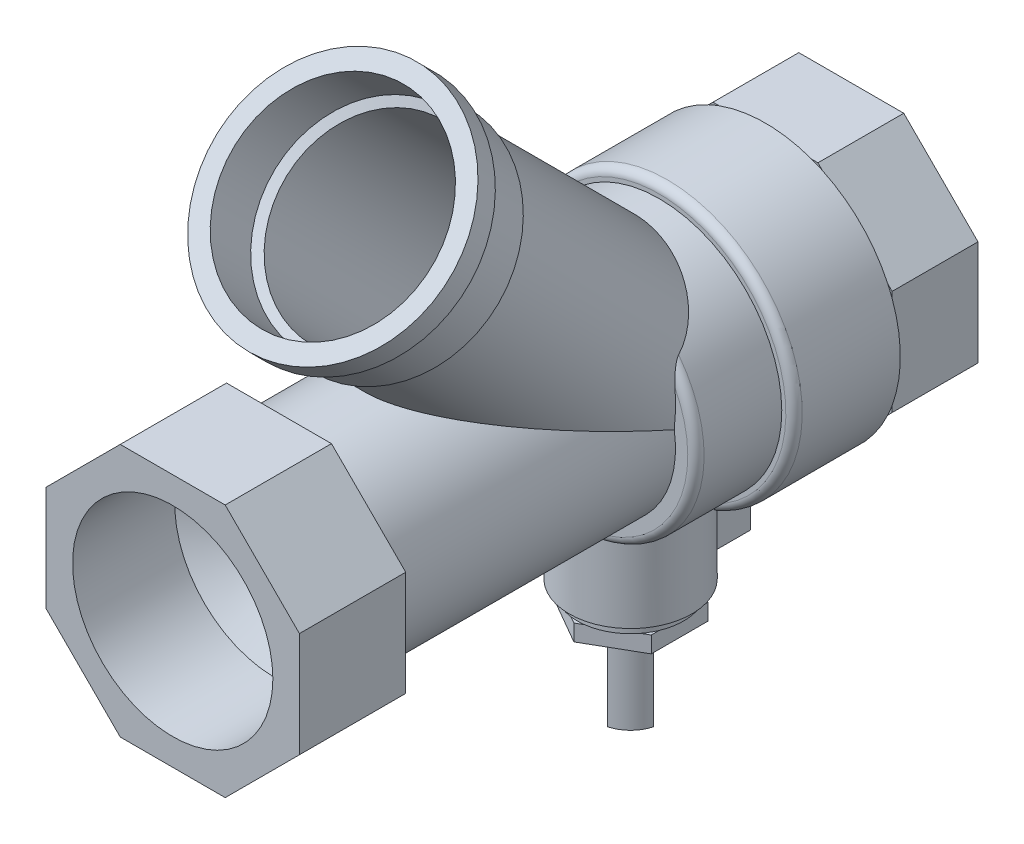
from build123d import *

# Parameters (mm, degrees)
SKETCH_1_R               = 15
EXTRUDE_1_DEPTH          = 10.5
SKETCH_2_R               = 12.5
EXTRUDE_2_DEPTH          = 36
EXTRUDE_3_DEPTH          = 13
SKETCH_4_R               = 16.5
EXTRUDE_4_DEPTH          = 13
EXTRUDE_5_DEPTH          = 10.5
FILLET_1_R               = 1
HOLE_WIZARD_G3_4_1_D     = 24.5
HOLE_WIZARD_G3_4_1_DEPTH = 12.5
HOLE_WIZARD_G3_4_1_TIP   = 7.360542583
HOLE_WIZARD_G3_4_2_D     = 24.5
HOLE_WIZARD_G3_4_2_DEPTH = 12.5
HOLE_WIZARD_G3_4_2_TIP   = 7.360542583
EXTRUDE_6_REACH          = 75.57
SKETCH_13_R              = 6.5
EXTRUDE_7_DEPTH          = 1.25
EXTRUDE_8_DEPTH          = 2
SKETCH_15_R              = 4
EXTRUDE_9_DEPTH          = 10
SKETCH_18_R              = 12.5
SKETCH_19_R              = 13.25
EXTRUDE_10_DEPTH         = 7
SKETCH_20_R              = 14.5
EXTRUDE_11_DEPTH         = 3
HOLE_WIZARD_G3_4_3_D     = 24.5
HOLE_WIZARD_G3_4_3_DEPTH = 7
HOLE_WIZARD_G3_4_3_TIP   = 7.360542583
SKETCH_24_R              = 11.25
CUT_EXTRUDE_2_DEPTH      = 45
CUT_EXTRUDE_1_REACH      = 97.54
SKETCH_11_R              = 7.5
CUT_EXTRUDE_START        = -10
CUT_EXTRUDE_3_DEPTH      = 10


with BuildPart() as part:
    # 草图1 → 凸台-拉伸1 (new body)
    with BuildSketch(Plane.XY):
        with Locations(Location((0, 0, 0), (0, 0, 180))):
            Circle(SKETCH_1_R)
    extrude(amount=EXTRUDE_1_DEPTH)

    # 草图2 → 凸台-拉伸2 (add)
    with BuildSketch(Plane.XY.offset(10.5)):
        Circle(SKETCH_2_R)
    extrude(amount=EXTRUDE_2_DEPTH)

    # 草图3 → 凸台-拉伸3 (add)
    with BuildSketch(Plane.XY.offset(46.5)):
        Polygon((6.420310217, -15.5), (15.5, -6.420310217), (15.5, 6.420310217), (6.420310217, 15.5), (-6.420310217, 15.5), (-15.5, 6.420310217), (-15.5, -6.420310217), (-6.420310217, -15.5), align=None)
    extrude(amount=EXTRUDE_3_DEPTH)

    # 草图4 → 凸台-拉伸4 (add)
    with BuildSketch(Plane(origin=(0, 0, 0), x_dir=(-1, 0, 0), z_dir=(0, 0, -1))):
        with Locations(Location((0, 0, 0), (0, 0, 180))):
            Circle(SKETCH_4_R)
    extrude(amount=EXTRUDE_4_DEPTH)

    # 草图6 → 凸台-拉伸5 (add)
    with BuildSketch(Plane(origin=(0, 0, -13), x_dir=(-1, 0, 0), z_dir=(0, 0, -1))):
        Polygon((15.5, -6.420310217), (15.5, 6.420310217), (6.420310217, 15.5), (-6.420310217, 15.5), (-15.5, 6.420310217), (-15.5, -6.420310217), (-6.420310217, -15.5), (6.420310217, -15.5), align=None)
    extrude(amount=EXTRUDE_5_DEPTH)

    # 圆角1
    fillet_1_edges = [part.edges().sort_by_distance(p)[0] for p in [
        (-16.5, 0, 0),
        (15, 0, 10.5),
    ]]
    fillet(fillet_1_edges, radius=FILLET_1_R)

    # G3/4 螺纹孔1
    with Locations(Plane.XY.offset(59.5)):
        with Locations((0, 0)):
            Hole(HOLE_WIZARD_G3_4_1_D / 2, depth=HOLE_WIZARD_G3_4_1_DEPTH)
            with Locations((0, 0, -(HOLE_WIZARD_G3_4_1_DEPTH + HOLE_WIZARD_G3_4_1_TIP / 2))):  # 118° drill point
                Cone(0, HOLE_WIZARD_G3_4_1_D / 2, HOLE_WIZARD_G3_4_1_TIP, mode=Mode.SUBTRACT)

    # G3/4 螺纹孔2
    with Locations(Plane(origin=(0, 0, -23.5), x_dir=(-1, 0, 0), z_dir=(0, 0, -1))):
        with Locations((0, 0)):
            Hole(HOLE_WIZARD_G3_4_2_D / 2, depth=HOLE_WIZARD_G3_4_2_DEPTH)
            with Locations((0, 0, -(HOLE_WIZARD_G3_4_2_DEPTH + HOLE_WIZARD_G3_4_2_TIP / 2))):  # 118° drill point
                Cone(0, HOLE_WIZARD_G3_4_2_D / 2, HOLE_WIZARD_G3_4_2_TIP, mode=Mode.SUBTRACT)

    # 草图12 → 凸台-拉伸6 (add, up to next)
    with BuildSketch(Plane(origin=(0, -23.5, 0), x_dir=(-1, 0, 0), z_dir=(0, -1, 0)), mode=Mode.PRIVATE) as extrude_6_sk1:
        with BuildLine():
            Line((-2.2, 9), (2.2, 9))
            Line((2.2, 9), (2.2, 3.670076708))
            ThreePointArc((2.2, 3.670076708), (0, -11), (-2.2, 3.670076708))
            Line((-2.2, 3.670076708), (-2.2, 9))
        make_face()
    extrude_6_tool1 = extrude(extrude_6_sk1.sketch, amount=-EXTRUDE_6_REACH, mode=Mode.PRIVATE) - part.part
    add(extrude_6_tool1.solids().sort_by_distance((0, -23.5, 2.377731))[0])

    # 草图13 → 凸台-拉伸7 (add)
    with BuildSketch(Plane.XZ.offset(23.5)):
        with Locations((0, 3.5)):
            Circle(SKETCH_13_R)
    extrude(amount=EXTRUDE_7_DEPTH)

    # 草图14 → 凸台-拉伸8 (add)
    with BuildSketch(Plane.XZ.offset(24.75)):
        Polygon((6, 6.964101615), (0, 10.42820323), (-6, 6.964101615), (-6, 0.035898385), (0, -3.42820323), (6, 0.035898385), align=None)
    extrude(amount=EXTRUDE_8_DEPTH)

    # 草图15 → 凸台-拉伸9 (add)
    with BuildSketch(Plane.XZ.offset(26.75)):
        with Locations((0, 3.5)):
            Circle(SKETCH_15_R)
    extrude(amount=EXTRUDE_9_DEPTH)

    # 扫描2: sweep along a path in 草图16
    with BuildLine(Plane(origin=(0, 0, 0), x_dir=(0, 0, -1), z_dir=(1, 0, 0))) as sweep_2_path:
        Line((-10.530023664, 0.160707832), (-35.118053174, 24.748737342))
    # 草图18 → 扫描2 (sweep)
    with BuildSketch(Plane(origin=(0, 5.345365748, 5.345365748), x_dir=(-0.9999999999999926, -8.68879538818696e-08, 8.688795429591137e-08), z_dir=(0, -0.7071067811865435, -0.7071067811865517))):
        with Locations((0, -4.117009359)):
            Circle(SKETCH_18_R)
    sweep(path=sweep_2_path.line)

    # 草图19 → 凸台-拉伸10 (add)
    with BuildSketch(Plane(origin=(0, 29.933395258, 29.933395258), x_dir=(1, 0, 0), z_dir=(0, 0.7071067811865434, 0.7071067811865517))):
        with Locations(Location((5.06e-07, -4.117009359, 0), (0, 0, 270))):
            Circle(SKETCH_19_R)
    extrude(amount=EXTRUDE_10_DEPTH)

    # 草图20 → 凸台-拉伸11 (add)
    with BuildSketch(Plane(origin=(0, 34.883142726, 34.883142726), x_dir=(1, 0, 0), z_dir=(0, 0.7071067811865434, 0.7071067811865517))):
        with Locations(Location((5.06e-07, -4.117009359, 0), (0, 0, 270))):
            Circle(SKETCH_20_R)
    extrude(amount=EXTRUDE_11_DEPTH)

    # G3/4 螺纹孔3
    with Locations(Plane(origin=(5.06e-07, 34.093297833, 39.915628305), x_dir=(0, 0.707106781187, -0.707106781187), z_dir=(0, 0.707106781187, 0.707106781187))):
        with Locations((0, 0)):
            Hole(HOLE_WIZARD_G3_4_3_D / 2, depth=HOLE_WIZARD_G3_4_3_DEPTH)
            with Locations((0, 0, -(HOLE_WIZARD_G3_4_3_DEPTH + HOLE_WIZARD_G3_4_3_TIP / 2))):  # 118° drill point
                Cone(0, HOLE_WIZARD_G3_4_3_D / 2, HOLE_WIZARD_G3_4_3_TIP, mode=Mode.SUBTRACT)

    # 草图24 → 切除-拉伸2 (cut)
    with BuildSketch(Plane(origin=(0, 37.004463069, 37.004463069), x_dir=(1, 0, 0), z_dir=(0, 0.7071067811865434, 0.7071067811865517))):
        with Locations(Location((5.06e-07, -4.117009359, 0), (0, 0, 270))):
            Circle(SKETCH_24_R)
    extrude(amount=-CUT_EXTRUDE_2_DEPTH, mode=Mode.SUBTRACT)

    # 切除-拉伸1: up to this cone (the profile starts outside it)
    cut_extrude_1_end = Plane(origin=(0, 0, -23.5), z_dir=(0, 0, 1)).offset(63.139458417) * Cone(1.664e-06, 58.084256944, 34.900541583, align=(Align.CENTER, Align.CENTER, Align.MIN), mode=Mode.PRIVATE)
    # 草图11 → 切除-拉伸1 (cut, up to the surface)
    with BuildSketch(Plane(origin=(0, 0, -23.5), x_dir=(-1, 0, 0), z_dir=(0, 0, -1)), mode=Mode.PRIVATE) as cut_extrude_1_sk1:
        Circle(SKETCH_11_R)
    cut_extrude_1_tool1 = extrude(cut_extrude_1_sk1.sketch, amount=-CUT_EXTRUDE_1_REACH, mode=Mode.PRIVATE) - cut_extrude_1_end
    add(cut_extrude_1_tool1.solids().sort_by_distance((0, 0, -23.5))[0], mode=Mode.SUBTRACT)

    # 草图25 → 切除-拉伸3 (cut)
    with BuildSketch(Plane.XZ.offset(36.75).offset(CUT_EXTRUDE_START)):
        with BuildLine():
            Line((1.03527618, 7.363703305), (-3.863703305, 2.46472382))
            ThreePointArc((-3.863703305, 2.46472382), (-2.828427125, 6.328427125), (1.03527618, 7.363703305))
        make_face()
        with BuildLine():
            Line((3.863703305, 4.53527618), (-1.03527618, -0.363703305))
            ThreePointArc((-1.03527618, -0.363703305), (2.828427125, 0.671572875), (3.863703305, 4.53527618))
        make_face()
    extrude(amount=CUT_EXTRUDE_3_DEPTH, mode=Mode.SUBTRACT)


solid = part.part
